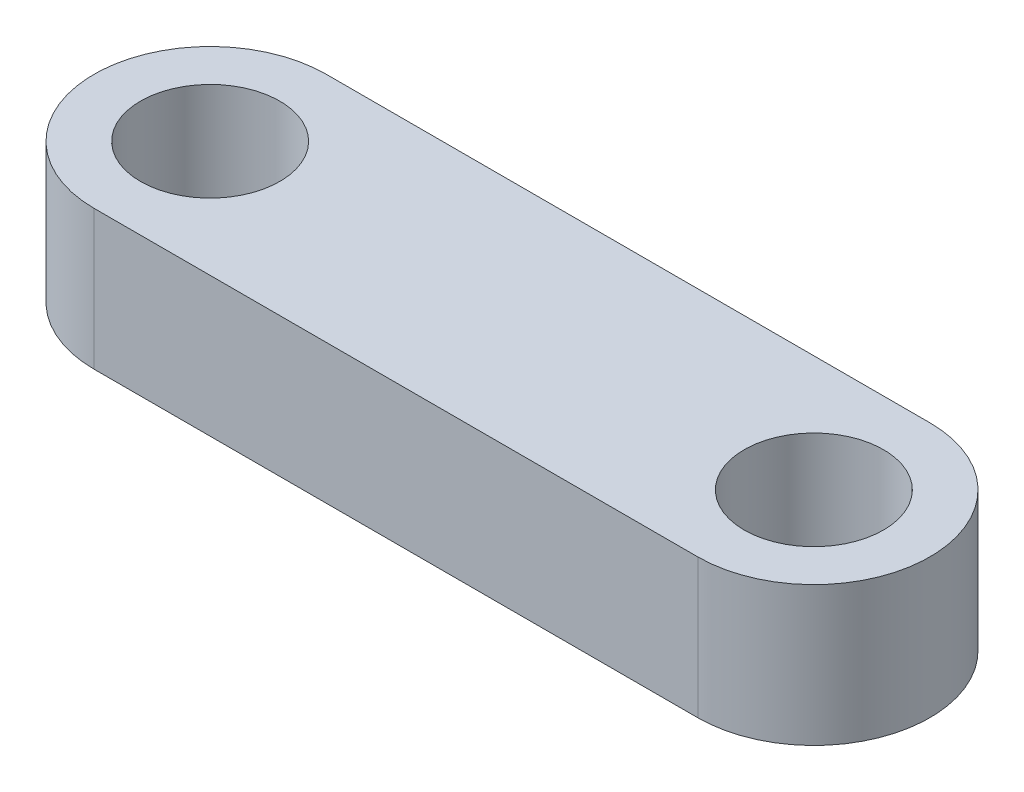
SolidWorks part; units mm, degrees
ref_plane "Front Plane" through (0, 0, 0) normal (0, 0, 1) x (1, 0, 0)
ref_plane "Top Plane" through (0, 0, 0) normal (0, 1, 0) x (1, 0, 0)
ref_plane "Right Plane" through (0, 0, 0) normal (1, 0, 0) x (0, 0, -1)
other "Configuration Table"
sketch "Sketch1" plane through (0, 0, 0) normal (0, 1, 0) x (1, 0, 0)
  line L0 (0, 0) -> (13, 0) construction
  line L1 (0, 2.5) -> (13, 2.5)
  line L2 (0, -2.5) -> (13, -2.5)
  arc A0 (0, 2.5) -> (0, -2.5) centre (0, 0) ccw
  arc A1 (13, -2.5) -> (13, 2.5) centre (13, 0) ccw
  circle A2 centre (0, 0) radius 1.5
  circle A3 centre (13, 0) radius 1.5
  point P3 (6.5, 0)
  dimension "D1" = 3
  dimension "D2" = 2.5
  dimension "10" = 13
extrude "Boss-Extrude1" add sketch "Sketch1" along normal blind 3
